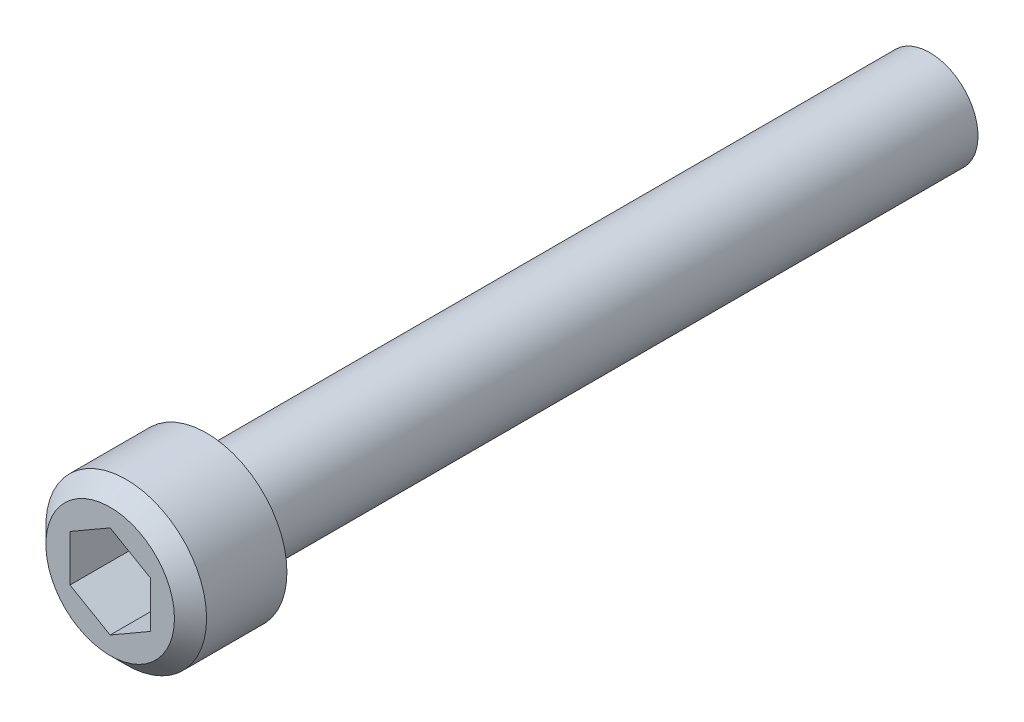
SolidWorks part; units mm, degrees
ref_plane "前视基准面" through (0, 0, 0) normal (0, 0, 1) x (1, 0, 0)
ref_plane "上视基准面" through (0, 0, 0) normal (0, 1, 0) x (1, 0, 0)
ref_plane "右视基准面" through (0, 0, 0) normal (1, 0, 0) x (0, 0, -1)
sketch "草图1" plane through (0, 0, 0) normal (0, 0, 1) x (1, 0, 0)
  circle A0 centre (0, 0) radius 5
  dimension "D1" = 10
extrude "凸台-拉伸1" add sketch "草图1" along normal blind 6
sketch "草图2" plane through (0, 0, 6) normal (0, 0, 1) x (1, 0, 0)
  line L1 (0, 2.8868) -> (-2.5, 1.4434)
  line L2 (-2.5, 1.4434) -> (-2.5, -1.4434)
  line L3 (-2.5, -1.4434) -> (0, -2.8868)
  line L4 (0, -2.8868) -> (2.5, -1.4434)
  line L5 (2.5, -1.4434) -> (2.5, 1.4434)
  line L6 (2.5, 1.4434) -> (0, 2.8868)
  circle A0 centre (0, 0) radius 2.5 construction
  dimension "D1" = 5
extrude "切除-拉伸1" cut sketch "草图2" against normal blind 4
chamfer "倒角1" distance 1 angle 45 1 edges at (5, 0, 6)
sketch "草图3" plane through (0, 0, 0) normal (0, 0, -1) x (-1, 0, 0)
  circle A0 centre (0, 0) radius 3
  dimension "D1" = 6
extrude "凸台-拉伸2" add sketch "草图3" along normal blind 45
cosmetic thread "装饰螺纹线1" parameters "D2"=4.917
